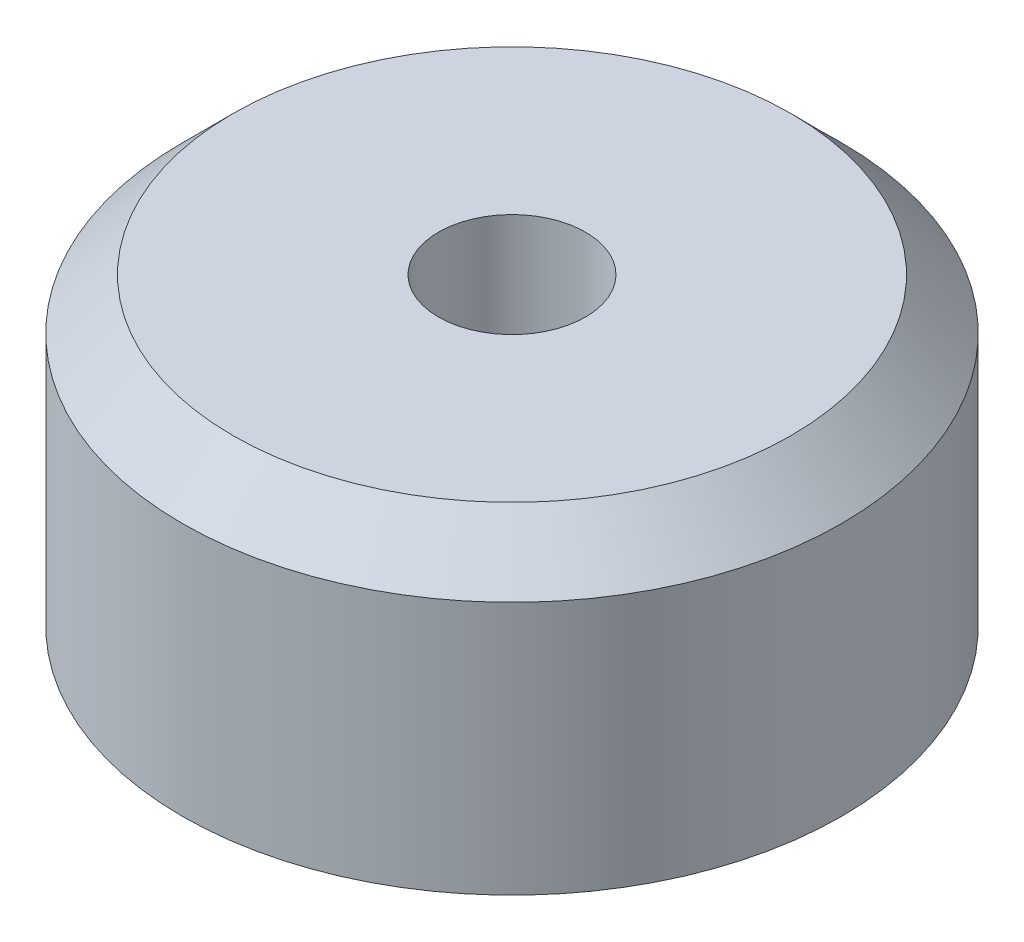
SolidWorks part; units mm, degrees
ref_plane "Front Plane" through (0, 0, 0) normal (0, 0, 1) x (1, 0, 0)
ref_plane "Top Plane" through (0, 0, 0) normal (0, 1, 0) x (1, 0, 0)
ref_plane "Right Plane" through (0, 0, 0) normal (1, 0, 0) x (0, 0, -1)
sketch "Sketch1" plane through (0, 0, 0) normal (0, 1, 0) x (1, 0, 0)
  circle A0 centre (0, 0) radius 32.5
  dimension "D1" = 65
extrude "Boss-Extrude1" add sketch "Sketch1" along normal blind 30
chamfer "Chamfer1" distance 5 angle 45 1 edges at (0, 30, 32.5)
hole_wizard "M16x1.5 Tapped Hole1" positions "Sketch2" profile "Sketch3" tap size "M16x1.5" standard "GB"
sketch "Sketch2" plane through (0, 30, 0) normal (0, 1, 0) x (1, 0, 0)
  point P0 (0, 0)
sketch "Sketch3" plane through (0, 30, 0) normal (1, 0, 0) x (0, 0, 1)
  line L0 (0, 0) -> (0, 40.8562)
  line L1 (0, 40.8562) -> (7.25, 36.5)
  line L2 (7.25, 36.5) -> (7.25, 0)
  line L5 (7.25, 0) -> (0, 0)
  line L10 (0, 40.8562) -> (-7.25, 36.5) construction
  line L11 (0, -6.35) -> (0, 107.95) construction
  dimension "螺纹孔钻头直径" = 14.5
  dimension "螺纹孔钻头深度" = 36.5
  dimension "导头角度" = 118
cosmetic thread "Hole Cosmetic Thread1"
